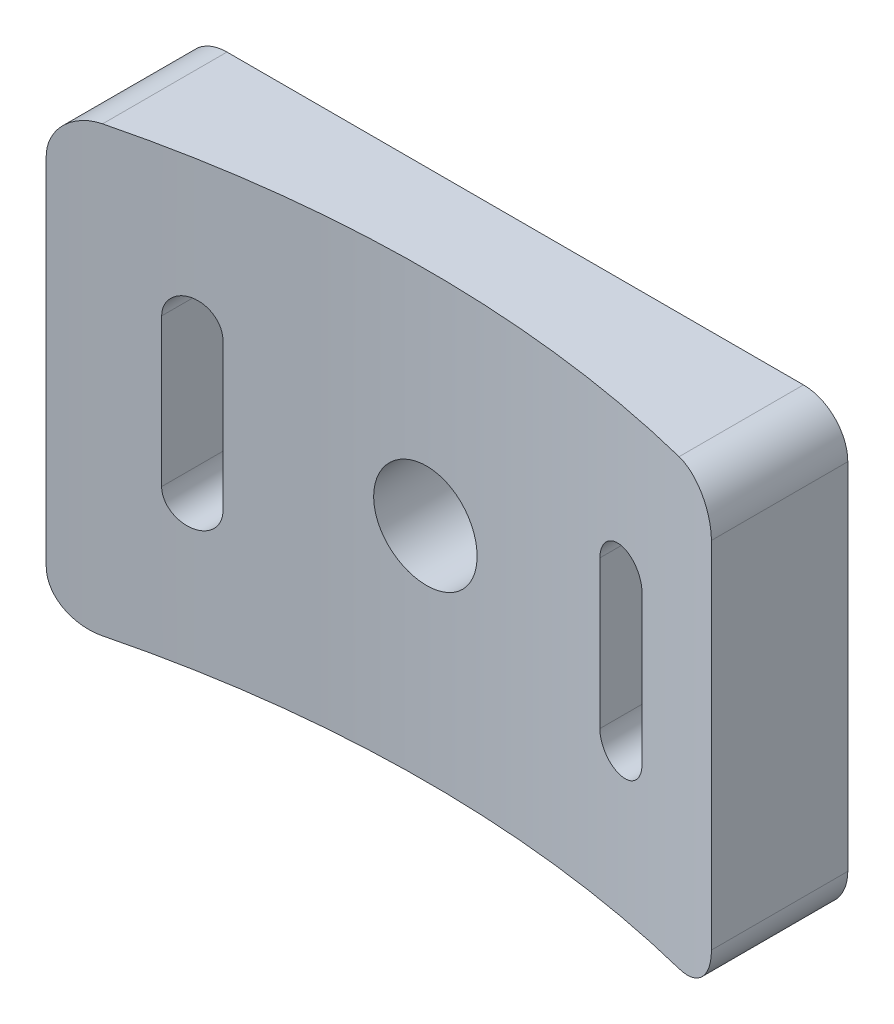
SolidWorks part; units mm, degrees
material "6061-T6 (SS)"
ref_plane "Front Plane" through (0, 0, 0) normal (0, 0, 1) x (1, 0, 0)
ref_plane "Top Plane" through (0, 0, 0) normal (0, 1, 0) x (1, 0, 0)
ref_plane "Right Plane" through (0, 0, 0) normal (1, 0, 0) x (0, 0, -1)
sketch "Sketch1" plane through (0, 0, 0) normal (0, 1, 0) x (1, 0, 0)
  line L0 (-22.5, 76.7708) -> (-22.5, 86)
  line L1 (-22.5, 86) -> (22.5, 86)
  line L2 (22.5, 86) -> (22.5, 76.7708)
  line L3 (0, 0) -> (0, 103.5063) construction
  arc A0 (22.5, 76.7708) -> (-22.5, 76.7708) centre (0, 0) ccw
  dimension "D1" = 160
  dimension "D2" = 45
  dimension "D4" = 86
extrude "Boss-Extrude1" add sketch "Sketch1" along normal blind 30
fillet "Fillet1" radius 3 4 edges at (-22.5, 0, -81.3854) (-22.5, 30, -81.3854) (22.5, 0, -81.3854) (22.5, 30, -81.3854)
hole_wizard "M8x1.0 Tapped Hole1" positions "Sketch3" profile "Sketch2" tap size "M8x1.0" standard "GB" end condition through all
sketch "Sketch3" plane through (0, 0, -86) normal (0, 0, -1) x (-1, 0, 0)
  line L0 (-19.5, 30) -> (19.5, 30) construction
  line L1 (-22.5, 27) -> (-22.5, 3) construction
  point P0 (0, 15)
  point P3 (0, 30)
  point P6 (-22.5, 15)
  dimension "D1" = 0
  dimension "D2" = 0
sketch "Sketch2" plane through (0, 15, -86) normal (1, 0, 0) x (0, 1, 0)
  line L0 (0, 0) -> (0, 9.4144)
  line L1 (0, 9.4144) -> (3.5, 9.4144)
  line L2 (3.5, 9.4144) -> (3.5, 0)
  line L5 (3.5, 0) -> (0, 0)
  line L11 (0, -6.35) -> (0, 107.95) construction
  dimension "通孔螺纹孔钻头直径" = 7
  dimension "通孔螺纹孔钻头深度" = 9.4144
cosmetic thread "Cosmetic Thread1" parameters "D2"=8
sketch "Sketch4" plane through (0, 0, -86) normal (0, 0, -1) x (-1, 0, 0)
  line L0 (-14.5, 20) -> (-14.5, 10) construction
  line L1 (-12.75, 20) -> (-12.75, 10)
  line L2 (-16.25, 20) -> (-16.25, 10)
  line L3 (14.5, 20) -> (14.5, 10) construction
  line L4 (16.25, 20) -> (16.25, 10)
  line L5 (12.75, 20) -> (12.75, 10)
  line L10 (0, 0) -> (0, 39.4662) construction
  line L11 (-22.5, 15) -> (30.8561, 15) construction
  line L12 (-22.5, 27) -> (-22.5, 3) construction
  arc A0 (-12.75, 20) -> (-16.25, 20) centre (-14.5, 20) ccw
  arc A1 (-16.25, 10) -> (-12.75, 10) centre (-14.5, 10) ccw
  arc A2 (16.25, 20) -> (12.75, 20) centre (14.5, 20) ccw
  arc A3 (12.75, 10) -> (16.25, 10) centre (14.5, 10) ccw
  point P2 (-14.5, 15)
  point P7 (14.5, 15)
  dimension "D5" = 1.75
  dimension "D6" = 1.75
  dimension "D1" = 29
  dimension "D3" = 10
  dimension "D4" = 10
extrude "Cut-Extrude1" cut sketch "Sketch4" against normal through all
sketch "Sketch5" plane through (0, 0, -86) normal (0, 0, -1) x (-1, 0, 0)
  line L0 (-14.5, 20) -> (-14.5, 10) construction
  line L1 (-11.5, 20) -> (-11.5, 10)
  line L2 (-17.5, 20) -> (-17.5, 10)
  line L3 (14.5, 20) -> (14.5, 10) construction
  line L4 (17.5, 20) -> (17.5, 10)
  line L5 (11.5, 20) -> (11.5, 10)
  arc A0 (-11.5, 20) -> (-17.5, 20) centre (-14.5, 20) ccw
  arc A1 (-17.5, 10) -> (-11.5, 10) centre (-14.5, 10) ccw
  arc A2 (17.5, 20) -> (11.5, 20) centre (14.5, 20) ccw
  arc A3 (11.5, 10) -> (17.5, 10) centre (14.5, 10) ccw
  point P2 (-14.5, 15)
  point P7 (14.5, 15)
  dimension "D1" = 3
  dimension "D2" = 3
extrude "Cut-Extrude2" cut sketch "Sketch5" against normal blind 3.3
